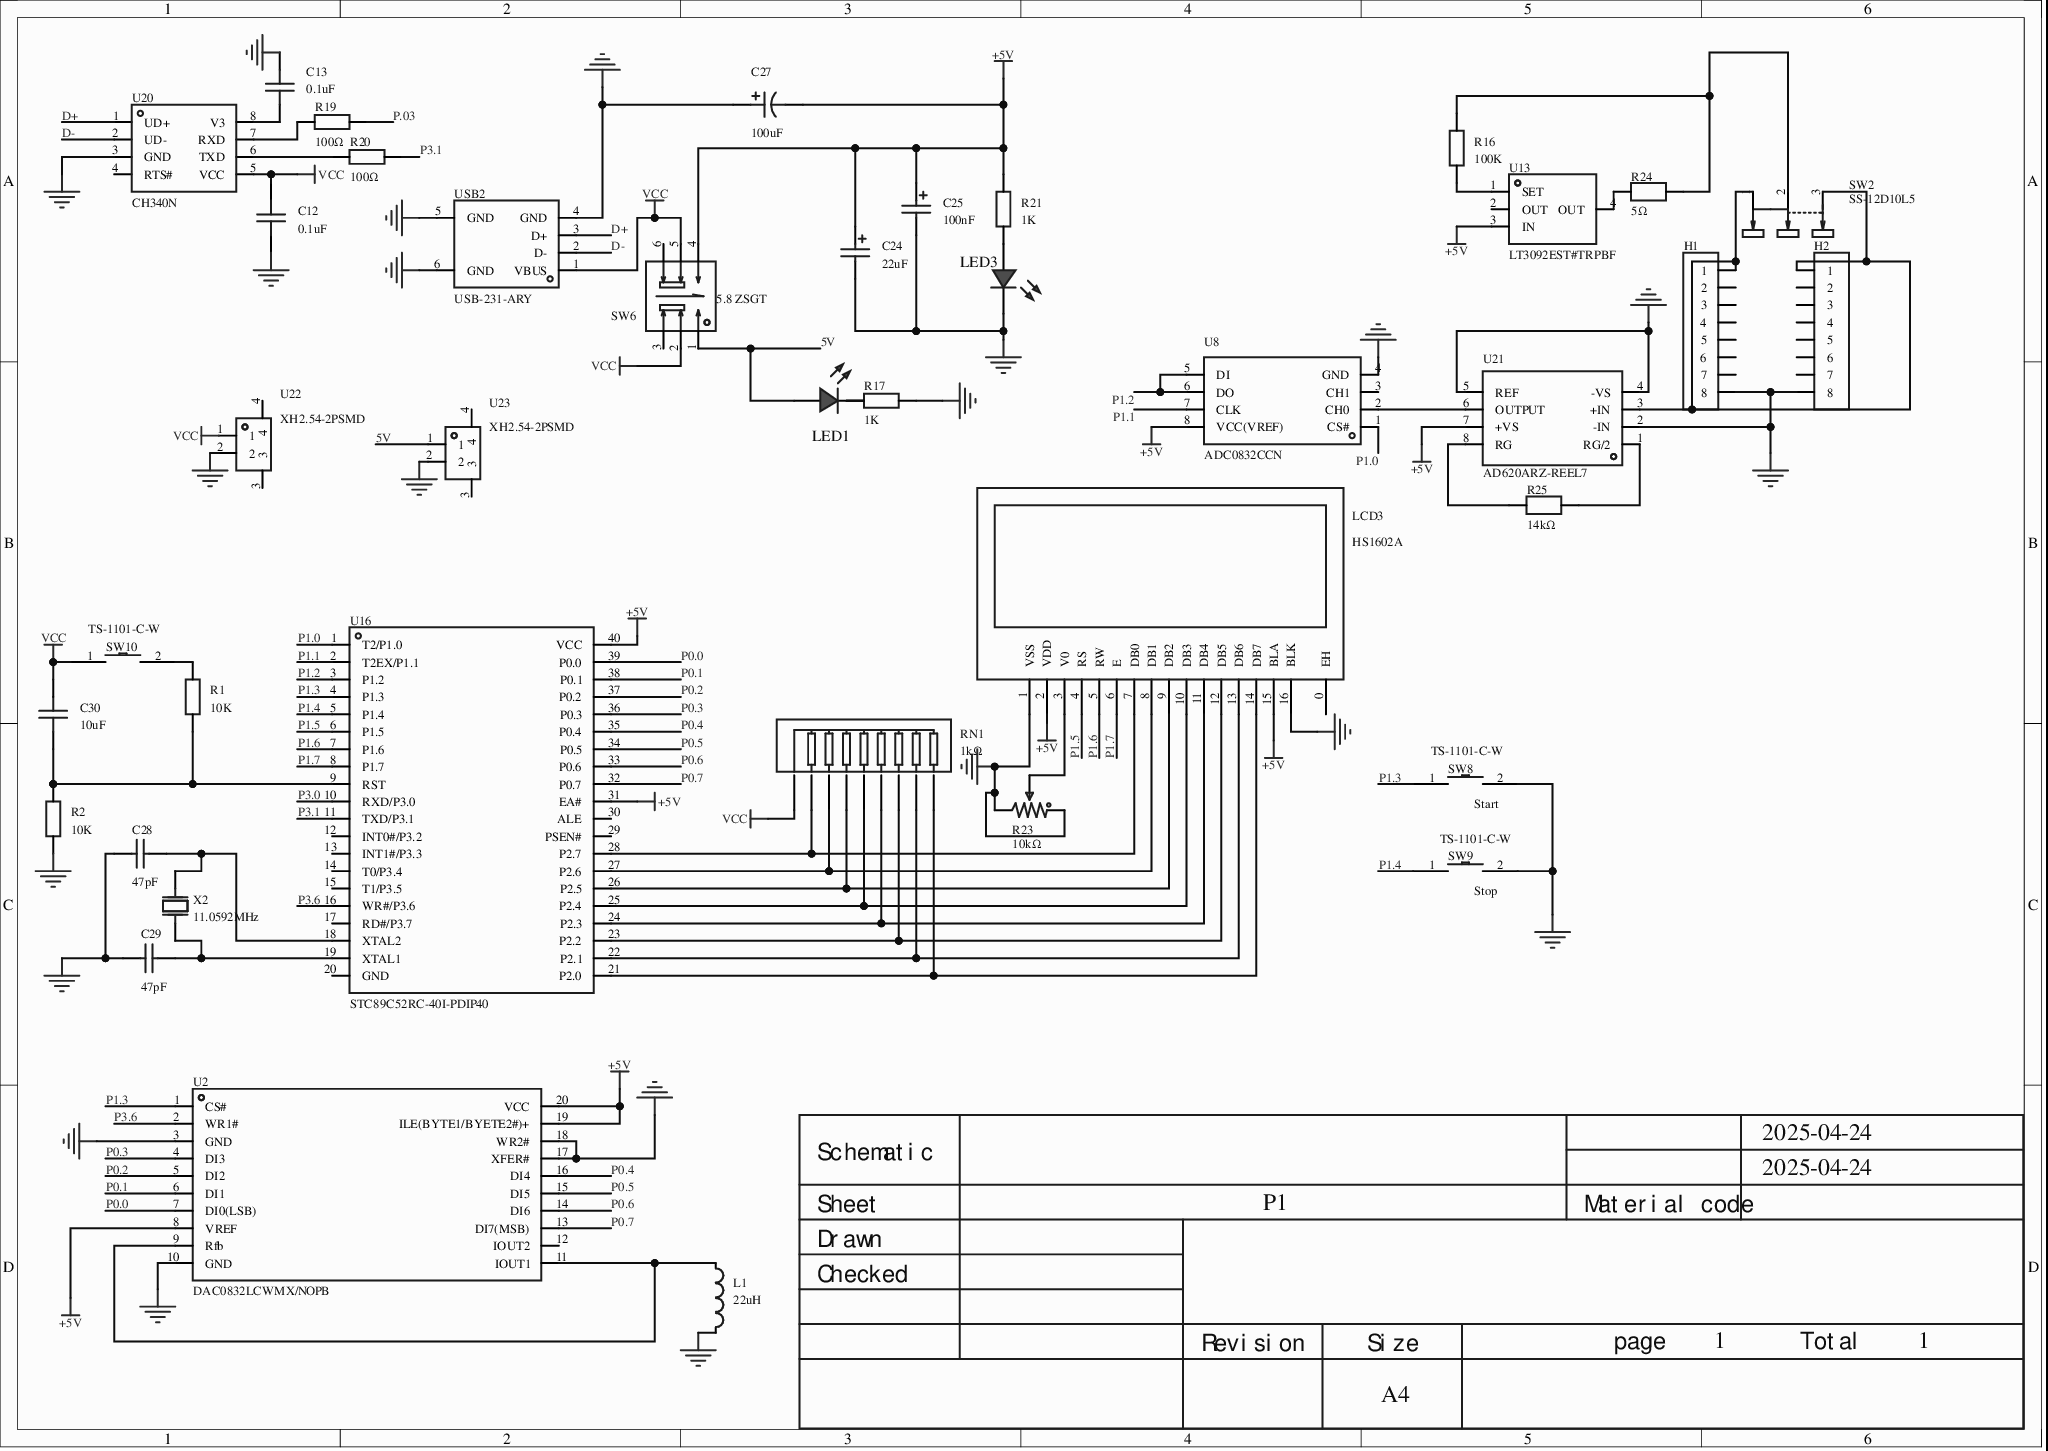
[diagram p0: MISC52088-3.schdoc]
# Altium project MISC52088-2.PrjPcb
1 sheet, 40 parts. Net scope: global (net labels, ports and power ports of the same name join across sheets).
Board file: MISC52088.pcbdoc

## Sheet MISC52088-3.schdoc
size 297 x 210 mm; Version: V1.0; @Project Name: MISC52088; @Page Count: 1; @Update Date: 2025-04-24; @Create Date: 2025-04-24; @Schematic Name: MISC52088; @Page No: 1; @Board Name: MISC52088; @Create Time: 22:25:30; @Update Time: 22:26:05

### Parts
C12  0.1uF  [C0603]
C13  0.1uF  [C0603]
C24  22uF  [CAP-SMD_L3.5-W2.8-R-RD]
C25  100nF  [CASE-A_3216]
C27  100uF  [CAP-SMD_BD8.1-L8.3-W8.3-LS9.3-FD]
C28  47pF  [C0603]
C29  47pF  [C0603]
C30  10uF  [C0603]
H1  (no value)  [HDR-TH_8P-P2.54-V-F-1]
H2  (no value)  [HDR-TH_8P-P2.54-V-F-1]
L1  22uH  [IND-TH_BD14.7-2P-P4.00]
LCD3  HS1602A  [LCD1602]
LED1  (no value)  [LED_0603]
LED3  (no value)  [LED_0603]
R1  10K  [R0603]
R2  10K  [R0603]
R16  100K  [R0603]
R17  1K  [R0603]
R19  100Ω  [R0603]
R20  100Ω  [R0603]
R21  1K  [R0603]
R23  10kΩ  [RES-ADJ-SMD_3P-L3.0-W3.8-P1.75-BR]
R24  5Ω  [R2512]
R25  14kΩ  [R0603]
RN1  1kΩ  [RES-ARRAY-TH_9P-P2.54-D1.0]
SW2  SS-12D10L5  [SW-TH_SS-12D10L5]
SW6  5.8 ZSGT  [SW-TH_5.8ZSGT]
SW8  TS-1101-C-W  [SW-SMD_L6.0-W3.3-LS8.0]
SW9  TS-1101-C-W  [SW-SMD_L6.0-W3.3-LS8.0]
SW10  TS-1101-C-W  [SW-SMD_L6.0-W3.3-LS8.0]
U2  DAC0832LCWMX/NOPB  [SOIC-20_L13.0-W7.6-P1.27-LS10.3-BL]
U8  ADC0832CCN  [DIP-8_L9.7-W6.4-P2.54-LS7.6-BL]
U13  LT3092EST#TRPBF  [SOT-223-4_L6.5-W3.5-P2.30-LS7.0-BR]
U16  STC89C52RC-40I-PDIP40  [DIP-40_L52.0-W13.7-P2.54-LS15.2-BL]
U20  CH340N  [SOP-8_L4.9-W3.9-P1.27-LS6.0-BL]
U21  AD620ARZ-REEL7  [SOIC-8_L5.0-W4.0-P1.27-LS6.0-BL]
U22  XH2.54-2PSMD  [CONN-SMD_XH2.54-2PSMD]
U23  XH2.54-2PSMD  [CONN-SMD_XH2.54-2PSMD]
USB2  USB-231-ARY  [USB-A-TH_USB-231-ARY]
X2  11.0592MHz  [HC-49US_L11.5-W4.5-P4.88]

### Nets
+5V: C24.1 C25.1 C27.2 LCD3.2(VDD) LCD3.15(BLA) R21.2 SW6.4 U2.8(VREF) U2.19(ILE(BYTE1/BYETE2#)+) U2.20(VCC) U8.8(VCC(VREF)) U13.3(IN) U16.31(EA#) U16.40(VCC) U21.7(+VS)
GND: C12.1 C13.1 C24.2 C25.2 C27.1 C28.1 C29.1 H1.8 H2.8 L1.2 LCD3.1(VSS) LCD3.16(BLK) LED3.1(C) R2.1 R17.2 R23.1 R23.3 SW8.2 SW9.2 U2.3(GND) U2.10(GND) U2.17(XFER#) U2.18(WR2#) U8.4(GND) U20.3(GND) U21.2(-IN) U21.4(-VS) U21.5(REF) U22.2 U23.2 USB2.4(GND) USB2.5(GND) USB2.6(GND)
VCC: C12.2 C30.2 RN1.1 SW6.2 SW6.5 SW10.1 U20.5(VCC) U22.1 USB2.1(VBUS)
5V: LED1.2(A) SW6.1 U23.1
D+: U20.1(UD+) USB2.3(D+)
D-: U20.2(UD-) USB2.2(D-)
P0.0: U2.7(DI0(LSB)) U16.39(P0.0)
P0.1: U2.6(DI1) U16.38(P0.1)
P0.2: U2.5(DI2) U16.37(P0.2)
P0.3: U2.4(DI3) U16.36(P0.3)
P0.4: U2.16(DI4) U16.35(P0.4)
P0.5: U2.15(DI5) U16.34(P0.5)
P0.6: U2.14(DI6) U16.33(P0.6)
P0.7: U2.13(DI7(MSB)) U16.32(P0.7)
P1.0: U8.1(CS#) U16.1(T2/P1.0)
P1.1: U8.7(CLK) U16.2(T2EX/P1.1)
P1.2: U8.5(DI) U8.6(DO) U16.3(P1.2)
P1.3: SW8.1 U2.1(CS#) U16.4(P1.3)
P1.4: SW9.1 U16.5(P1.4)
P1.5: LCD3.4(RS) U16.6(P1.5)
P1.6: LCD3.5(RW) U16.7(P1.6)
P1.7: LCD3.6(E) U16.8(P1.7)
P3.0: U16.10(RXD/P3.0)
P3.1: R20.2 U16.11(TXD/P3.1)
P3.6: U2.2(WR1#) U16.16(WR#/P3.6)
P.03: R19.2
NetC13_2: C13.2 U20.8(V3)
NetC28_2: C28.2 U16.18(XTAL2) X2.1(OSC1)
NetC29_2: C29.2 U16.19(XTAL1) X2.2(OSC2)
NetC30_1: C30.1 R1.1 R2.2 U16.9(RST)
NetH1_1: H1.1 H2.1 SW2.1 SW2.3 U21.3(+IN)
NetL1_1: L1.1 U2.9(Rfb) U2.11(IOUT1)
NetLCD3_3: LCD3.3(V0) R23.2
NetLCD3_7: LCD3.7(DB0) RN1.2 U16.28(P2.7)
NetLCD3_8: LCD3.8(DB1) RN1.3 U16.27(P2.6)
NetLCD3_9: LCD3.9(DB2) RN1.4 U16.26(P2.5)
NetLCD3_10: LCD3.10(DB3) RN1.5 U16.25(P2.4)
NetLCD3_11: LCD3.11(DB4) RN1.6 U16.24(P2.3)
NetLCD3_12: LCD3.12(DB5) RN1.7 U16.23(P2.2)
NetLCD3_13: LCD3.13(DB6) RN1.8 U16.22(P2.1)
NetLCD3_14: LCD3.14(DB7) RN1.9 U16.21(P2.0)
NetLED1_1: LED1.1(C) R17.1
NetLED3_2: LED3.2(A) R21.1
NetR1_2: R1.2 SW10.2
NetR16_1: R16.1 U13.1(SET)
NetR16_2: R16.2 R24.2 SW2.2
NetR19_1: R19.1 U20.7(RXD)
NetR20_1: R20.1 U20.6(TXD)
NetR24_1: R24.1 U13.4(OUT)
NetR25_1: R25.1 U21.8(RG)
NetR25_2: R25.2 U21.1(RG/2)
NetU8_2: U8.2(CH0) U21.6(OUTPUT)

Not connected (* = marked no-connect by the designer): H1 2 3 4 5 6 7; H2 2 3 4 5 6 7; LCD3 0(EH); SW6 3 6; U2 12(IOUT2); U8 3(CH1); U13 2(OUT); U16 12(INT0#/P3.2) 13(INT1#/P3.3) 14(T0/P3.4) 15(T1/P3.5) 17(RD#/P3.7) 20(GND) 29(PSEN#) 30(ALE); U20 4(RTS#); U22 3 4; U23 3 4

### Notes on the sheet
- (near SW8) Start
- (near SW9) Stop
- 2025-04-24
- Schematic
- Sheet
- P1
- Material code
- Checked
- Drawn
- Revision
- Size
- A4
- page
- 1
- Total

### Library data of the parts
C12 C13 = CAP_0603: ConvertToPcb: yes; SymbolName: CapAcitance; ModelId: ac125912035d415993ca9572d50418b1; ModelName: C0603_L1.6-W0.8-H0.8; ModelTransform: 62.992,31.496,0,0,0,0,0,0,0; Value: 100nF; Device: CAP_0603; AddInBom: yes; Supplier Footprint: 0603; FootprintName: C0603
C24 = 6TPE220MAZB: Capacitance: 220uF; tolerance: ±20%; rated voltage: 6.3V; equivalent series resistance (ESR): 35mΩ@100kHz;; Manufacturer: PANASONIC(松下); AddInBom: yes; ModelId: 0dfcda272f9b43668c6086d3a08712ba; ModelName: CASE-B_L3.5-W2.8-H1.9; ModelTransform: 145.669,110.236,0,180,0,0,0,0,0; Symbol: 6TPE220MAZB; Value: 22uF; Device: 6TPE220MAZB; LCSC Part Name: 220uF ±20% 6.3V MSL=3拆包后请尽快使用; ManufacturerPart: 6TPE220MAZB; Supplier Footprint: -; JLCPCB Part Class: Extended library; Datasheet: https://atta.szlcsc.com/upload/public/pdf/source/20180301/C178383_15198943937361383951.pdf; Supplier: LCSC; ConvertToPcb: yes; FootprintName: CAP-SMD_L3.5-W2.8-R-RD; Tolerance: ±20%; Voltage Rating: 6.3V; Equivalent Series Resistance(ESR): 35mΩ@100kHz; Operating Temperature: -55℃~+105℃
C25 = TAJA104K035RNJ: Capacitance: 100nF; tolerance: ±10%; rated voltage: 35V; equivalent series resistance: 24Ω@100kHz;; Manufacturer: Kyocera AVX; AddInBom: yes; ModelId: 803ac3def75e4c7cb895540fe23dd6a1; ModelTransform: 125.984,62.992,0,0,0,0,0,0,0; Symbol: TAJA104K035RNJ; Device: TAJA104K035RNJ; LCSC Part Name: 100nF ±10% 35V; SupplierPart: C7173; ManufacturerPart: TAJA104K035RNJ; Supplier Footprint: CASE-A-3216; JLCPCB Part Class: Extended library; Datasheet: https://atta.szlcsc.com/upload/public/pdf/source/20160107/1457707750344.pdf; Supplier: LCSC; ConvertToPcb: yes; FootprintName: CASE-A_3216; ModelName: CASE-A_3216; Value: 100nF; Tolerance: ±10%; Rated Voltage: 35V; Equivalent Series Resistance(ESR): 24Ω@100kHz; Operating Temperature: -55℃~+125℃
C27 = GVE1H107M0810CNVC: Capacitance: 100uF; tolerance: ±20%; rated voltage: 50V; ripple current: 300mA@100kHz; equivalent series resistance: 600mΩ@100kHz;; Manufacturer: HRK(鸿瑞凯电子); AddInBom: yes; ModelId: 42ed741c1b0b4e9db37bf14bd0fb5205; ModelTransform: 354.33,326.771,0,180,0,0,0,0,0; φD: 8mm; L: 10.5mm; Lifetime @ Temp: 2000hrs@105℃; Symbol: GVE1H107M0810CNVC; Device: GVE1H107M0810CNVC; LCSC Part Name: 100uF ±20% 50V; SupplierPart: C2983307; ManufacturerPart: GVE1H107M0810CNVC; Supplier Footprint: SMD,D8xL10.5mm; JLCPCB Part Class: Extended library; Datasheet: https://atta.szlcsc.com/upload/public/pdf/source/20220321/B5A059027F69866A3EEEBC781A889613.pdf; Supplier: LCSC; ConvertToPcb: yes; FootprintName: CAP-SMD_BD8.1-L8.3-W8.3-LS9.3-FD; ModelName: CAP-SMD_BD8.1-L8.3-W8.3-LS9.3-FD; Value: 100uF; Tolerance: ±20%; Rated Voltage: 50V; Ripple Current: 300mA@100kHz; Equivalent Series Resistance(ESR): 600mΩ@100kHz; Operating Temperature: -55℃~+105℃
C28 C29 = CL10C470JB8NNNC: Capacitance: 47pF; tolerance: ±5%; rated voltage: 50V; dielectric (temperature coefficient): C0G;; Manufacturer: SAMSUNG(三星); AddInBom: yes; ModelId: ac125912035d415993ca9572d50418b1; ModelName: C0603_L1.6-W0.8-H0.8; ModelTransform: 62.992,31.496,0,0,0,0,0,0,0; Symbol: CL10C470JB8NNNC; Device: CL10C470JB8NNNC; LCSC Part Name: 47pF ±5% 50V; SupplierPart: C1671; ManufacturerPart: CL10C470JB8NNNC; Supplier Footprint: 0603; JLCPCB Part Class: Basic library; Datasheet: https://atta.szlcsc.com/upload/public/pdf/source/20160218/1457707763339.pdf; Supplier: LCSC; ConvertToPcb: yes; FootprintName: C0603; Value: 47pF; Tolerance: ±5%; Voltage Rated: 50V; Temperature Coefficient: C0G
C30 = CGA0603X5R106K100JT: Capacitance: 10uF; tolerance: ±10%; rated voltage: 10V; temperature coefficient: X5R;; Manufacturer: HRE(芯声); AddInBom: yes; ModelId: ac125912035d415993ca9572d50418b1; ModelName: C0603_L1.6-W0.8-H0.8; ModelTransform: 62.992,31.496,0,0,0,0,0,0,0; Symbol: CGA0603X5R106K100JT; Device: CGA0603X5R106K100JT; LCSC Part Name: 10uF ±10% 10V; SupplierPart: C6119842; ManufacturerPart: CGA0603X5R106K100JT; Supplier Footprint: 0603; JLCPCB Part Class: Extended library; Supplier: LCSC; ConvertToPcb: yes; FootprintName: C0603; Value: 10uF; Tolerance: ±10%; Voltage Rating: 10V; Temperature Coefficient: X5R
H1 H2 = HDR-F_2.54_1x8P: Symbol: Header-Female-2.54_1x8; AddInBom: yes; ModelId: 0f7e4d9227ef4fa08d5469c22cc70cdb; ModelName: HDR-F-2.54_1x8; ModelTransform: 799.99844,100,0,0,0,0,0,0,-118.11; Device: HDR-F_2.54_1x8P; ConvertToPcb: yes; FootprintName: HDR-TH_8P-P2.54-V-F-1; SupplierPart: C27438; Supplier Footprint: 插件
L1 = PDMTAT044125-220MWU: Inductance: 22uH; tolerance: ±20%; rated current: 8A; saturation current (Isat): -; type: toroidal inductor; Q factor: -;; Manufacturer: PROD(谱罗德); AddInBom: yes; ModelId: ffc1d1e6ac7e4445805eb288369d3ccc; ModelTransform: 578.23735,577.65514,0,0,0,0,0,196.85,-118.11; DC Resistance: 15mΩ; Symbol: PDMTAT044125-220MWU; Device: PDMTAT044125-220MWU; LCSC Part Name: 磁环电感 22uH ±20%; SupplierPart: C2909799; ManufacturerPart: PDMTAT044125-220MWU; Supplier Footprint: 插件,D=14.5mm; JLCPCB Part Class: Extended library; Datasheet: https://atta.szlcsc.com/upload/public/pdf/source/20211105/260D4E3EA41F790233DE2825ED13716B.pdf; Supplier: LCSC; ConvertToPcb: yes; FootprintName: IND-TH_BD14.7-2P-P4.00; ModelName: IND-TH_BD14.7-2P-P4.00; Value: 22uH; Tolerance: ±20%; Rated Current: 8A; Current - Saturation (Isat): -; Type: Toroidal inductor; Q @ Frequency: -; Frequency - Self Resonant: -; Ratings: AEC-Q200
LCD3 = HS1602A: Controller chip: SPLC780; size (inch): 2;; Manufacturer: HS(汉昇); AddInBom: yes; ModelId: f9d832f46a914cadb50fc4d4cefd2517; ModelTransform: 3149.6,1417.32,0,0,0,0,0,0,-118.11; Symbol: HS1602A; Device: HS1602A; LCSC Part Name: 2.0寸16*2单色字符字符液晶显示屏; SupplierPart: C5329588; ManufacturerPart: HS1602A; Supplier Footprint: -; JLCPCB Part Class: Extended library; Datasheet: https://atta.szlcsc.com/upload/public/pdf/source/20221212/35734F14DBB323F90DD8DBE1717CD9FD.pdf; Supplier: LCSC; ConvertToPcb: yes; FootprintName: LCD1602; ModelName: LCD1602; Main Control Chip: SPLC780; Size: 2; Operating Temperature: -20℃~+70℃
LED1 LED3 = LED_0603-R: Symbol: LED_R; Convert to PCB: yes; 3D Model: dd8257b0d61a4cd7b68939a056e08095; 3D Model Transform: 58.72,29.4,22.03,0,0,0,0,0,0; ModelName: LED-0603_R; Device: LED_0603-R; Add into BOM: yes; Supplier Footprint: 0603; FootprintName: LED_0603
R1 R2 R21 = Res_0603: ConvertToPcb: yes; SymbolName: Resistor; ModelId: fc143cca1e79419f9cd78b61e9279f08; ModelTransform: 31.8897,63.7794,0,90,0,0,0,0,0; Device: Res_0603; AddInBom: yes; Supplier Footprint: 0603; FootprintName: R0603; ModelName: R0603
  R1 R2: Value: 10K
  R21: Value: 1K
R16 R17 R19 R20 = Res_0603: ConvertToPcb: yes; SymbolName: Resistor; ModelId: fc143cca1e79419f9cd78b61e9279f08; ModelTransform: 31.8897,63.7794,0,90,0,0,0,0,0; Value: 10K; Device: Res_0603; AddInBom: yes; Supplier Footprint: 0603; FootprintName: R0603; ModelName: R0603
R23 = TC33X-2-103E: Resistance: 10kΩ; tolerance: ±25%; power: 150mW; temperature coefficient: ±250ppm/℃;; Manufacturer: BOURNS; AddInBom: yes; ModelId: 6fe475bd84584852aea8190beccbfb0a; ModelTransform: 118.11,150,0,90,0,0,4.882,0,0; Turns: 1; Symbol: TC33X-2-103E; Device: TC33X-2-103E; LCSC Part Name: 10kΩ ±25%; SupplierPart: C719176; ManufacturerPart: TC33X-2-103E; Supplier Footprint: SMD-3P,3.8x3.6mm; JLCPCB Part Class: Extended library; Datasheet: https://atta.szlcsc.com/upload/public/pdf/source/20200810/C720646_BB66A75E654D5E1D30127FF45BCD3C26.pdf; Supplier: LCSC; ConvertToPcb: yes; FootprintName: RES-ADJ-SMD_3P-L3.0-W3.8-P1.75-BR; ModelName: RES-ADJ-SMD_3P-L3.0-W3.8-P1.75-BR; Value: 10kΩ; Tolerance: ±25%; Rated Voltage: -; Power(Watts): 150mW; Temperature Coefficient: ±250ppm/℃
R24 = HoAR2512-1W-5R-0.1%-TCR25: Resistor type: ceramic resistor; resistance: 5Ω; tolerance: ±0.1%; power: 1W; temperature coefficient: ±25ppm/℃;; Manufacturer: Milliohm(毫欧); AddInBom: yes; ModelId: 954b67263d9e4f3582d8de3f8c846421; ModelName: R2512_L6.3-W3.2-H0.6; ModelTransform: 248.031,125.984,0,0,0,0,-0.0005,0,0; Symbol: HOAR2512-1W-5R-0.1%-TCR25; Device: HoAR2512-1W-5R-0.1%-TCR25; LCSC Part Name: 陶瓷电阻 5Ω ±0.1% 1W; SupplierPart: C5123609; ManufacturerPart: HoAR2512-1W-5R-0.1%-TCR25; Supplier Footprint: 2512; JLCPCB Part Class: Extended library; Datasheet: https://atta.szlcsc.com/upload/public/pdf/source/20220805/BC8894D01B21B12D20FF0E940066DD50.pdf; Supplier: LCSC; ConvertToPcb: yes; FootprintName: R2512; Type: Ceramic resistor; Value: 5Ω; Tolerance: ±0.1%; Power(Watts): 1W; Temperature Coefficient: ±25ppm/℃
R25 = FRC0603F1402TS: Resistor type: thick-film resistor; resistance: 14kΩ; tolerance: ±1%; power: 100mW; operating voltage: 75V; temperature coefficient: ±100ppm/℃;; Manufacturer: FOJAN(富捷); AddInBom: yes; ModelId: fc143cca1e79419f9cd78b61e9279f08; ModelTransform: 31.8897,63.7794,0,90,0,0,0,0,0; Symbol: FRC0603F1402TS; Device: FRC0603F1402TS; LCSC Part Name: 14kΩ ±1% 100mW 厚膜电阻; SupplierPart: C2930066; ManufacturerPart: FRC0603F1402TS; Supplier Footprint: 0603; JLCPCB Part Class: Extended library; Datasheet: https://atta.szlcsc.com/upload/public/pdf/source/20211221/925EC7D7225764EE0046F22065062C87.pdf; Supplier: LCSC; ConvertToPcb: yes; FootprintName: R0603; ModelName: R0603; Type: Thick-film resistor; Value: 14kΩ; Tolerance: ±1%; Power(Watts): 100mW; Voltage-Supply(Max): 75V; Temperature Coefficient: ±100ppm/℃; Operating Temperature: -55℃~+155℃
RN1 = A09-102JP: Number of resistors: 8; resistance: 1kΩ; tolerance: ±5%; power per element: 125mW; temperature coefficient: ±100ppm/℃;; Manufacturer: FH(风华); AddInBom: yes; ModelId: d106c67f29e14d8080ba548247a719a1; ModelName: SIP-9_L22.8-W3.0-H8.5-P2.54; ModelTransform: 917.49722,118.11,0,0,0,0,0,0,-137.795; Number of Resistors: 8; Symbol: A09-102JP; Device: A09-102JP; LCSC Part Name: 1kΩ ±5%; SupplierPart: C9111; ManufacturerPart: A09-102JP; Supplier Footprint: SIP-9-2.54mm; JLCPCB Part Class: Extended library; Datasheet: https://atta.szlcsc.com/upload/public/pdf/source/20181127/C336620_2E84FA9E7B5BF76546BC661699514FB8.pdf; Supplier: LCSC; ConvertToPcb: yes; FootprintName: RES-ARRAY-TH_9P-P2.54-D1.0; Value: 1kΩ; Tolerance: ±5%; Power(Watts): 125mW; Temperature Coefficient: ±100ppm/℃; Number of Pins: 9
SW2 = SS-12D10L5: Circuit structure: SPDT; mounting: through-hole; switch colour: black; rated current (DC): 3A; rated voltage (DC): 125V; rated current (AC): 3A; rated voltage (AC): 125V; mechanical life: 1 ten-thousand cycles;; Manufacturer: XKB Connectivity(中国星坤); AddInBom: yes; ModelId: c49f07a32c154ec8ad7cf47670a53981; ModelName: SW-TH_L13.0-W6.8-H6.4-P4.7; ModelTransform: 511.81,267.716,0,0,0,0,0,0,-275.591; Actuator Style: Rectangular post; Pin Style: PC pin; Switch Length: 13mm; Switch Width: 6.8mm; Switch Height: 6.4mm; Symbol: SS-12D10L5; Device: SS-12D10L5; LCSC Part Name: 柄长5mm 直插双档 滑动开关; SupplierPart: C319012; ManufacturerPart: SS-12D10L5; Supplier Footprint: 插件; JLCPCB Part Class: Extended library; Datasheet: https://atta.szlcsc.com/upload/public/pdf/source/20211009/D6412F37AABE6F9459A6EE7FA4DAEADB.pdf; Supplier: LCSC; ConvertToPcb: yes; FootprintName: SW-TH_SS-12D10L5; Circuit: SPDT; Mounting Style: Through-hole; Actuator Color: Black; Current Rating (DC): 3A; Voltage Rating (DC): 125V; Current Rating (AC): 3A; Voltage Rating (AC): 125V; Mechanical Life: 1 ten-thousand cycles; Operating Temperature: -40℃~+85℃
SW6 = 5.8 ZSGT: Circuit structure: DPDT; self-lock / no-lock: self-lock; mounting: through-hole; contact current: 110mA; rated voltage (DC): 30V; with lamp: without; actuating force: 1.5N; mechanical life: 10 ten-thousand cycles;; Manufacturer: SHOU HAN(首韩); AddInBom: yes; ModelId: 3b6e980975cd43bda015b2e9aaa869d3; ModelTransform: 228.346,228.346,0,0,0,0,0,0,-141.732; Actuator Style: Square button; Insulation Resistance: 100MΩ; Actuator/Cap Color: White; Pin Style: PC pin; Symbol: 5.8 ZSGT; Device: 5.8 ZSGT; LCSC Part Name: 5.8*5.8有头/高头 带锁/自锁开关 泡泡机开关; SupplierPart: C2681587; ManufacturerPart: 5.8 ZSGT; Supplier Footprint: 插件; JLCPCB Part Class: Extended library; Datasheet: https://atta.szlcsc.com/upload/public/pdf/source/20210107/C2681587_CDDDDA4A1C7AC9FEB01815B75893A6BA.pdf; Supplier: LCSC; ConvertToPcb: yes; FootprintName: SW-TH_5.8ZSGT; ModelName: SW-TH_5.8ZSGT; Circuit: DPDT; Self Lock / No Lock: Self-lock; Mounting Style: Through-hole; Contact Current: 110mA; Voltage Rating (DC): 30V; With Lamp: Without; Operating Force: 1.5N; Operating Temperature: -10℃~+70℃; Mechanical Life: 10 ten-thousand cycles
SW8-SW10 = TS-1101-C-W: Circuit structure: SPST; button shape: rectangular button; actuating force: 260gf; mounting: surface mount; switch length: 6mm; switch width: 3.6mm; switch height: 2.5mm; with bracket: without; contact current: 50mA; rated voltage (AC): -; rated voltage (DC): 12V; rated power: -; insulation resistance: -; with lamp: none; mechanical life: 5 ten-thousand cycles;; Manufacturer: XKB Connectivity(中国星坤); AddInBom: yes; ModelId: b2f4ea9f0afc4b0786d53dba66ceb9e4; ModelName: SW-SMD_L6.0-W3.3-H5-LS8.0; ModelTransform: 314.96,129.921,0,0,0,0,0,0,0; Actuator/Cap Color: White with light green; Symbol: TS-1101-C-W; Device: TS-1101-C-W; LCSC Part Name: 6*3.6*2.5mm 立贴 轻触开关; SupplierPart: C318938; ManufacturerPart: TS-1101-C-W; Supplier Footprint: SMD; JLCPCB Part Class: Extended library; Datasheet: https://atta.szlcsc.com/upload/public/pdf/source/20200227/C318938_C2E53B1EEDE37D980A33616AC086DE53.pdf; Supplier: LCSC; ConvertToPcb: yes; FootprintName: SW-SMD_L6.0-W3.3-LS8.0; Circuit: SPST; Actuator Style: Rectangular button; Operating Force: 260gf; Mounting Style: Surface mount; Switch Length: 6mm; Switch Width: 3.6mm; Switch Height: 2.5mm; Strike Gundam: Without; Contact Current: 50mA; Voltage Rating (AC): -; Voltage Rating (DC): 12V; Power Rating: -; Insulation Resistance: -; With Lamp: None; IP Rating: -; Pin Style: -; Mechanical Life: 5 ten-thousand cycles; Operating Temperature: -30℃~+85℃
U2 = DAC0832LCWMX/NOPB: Manufacturer: TI(德州仪器); AddInBom: yes; ModelId: fc022553ecdc4755a737d639ae95109c; ModelName: SOIC-20_L12.8-W7.5-H2.7-LS10.3-P1.27; ModelTransform: 503.936,409.68154,0,0,0,0,0,0,0; Symbol: DAC0832LCWMX/NOPB; Device: DAC0832LCWMX/NOPB; LCSC Part Name: DAC0832LCWMX/NOPB; SupplierPart: C17194366; ManufacturerPart: DAC0832LCWMX/NOPB; Supplier Footprint: SOIC-20; JLCPCB Part Class: Extended library; Supplier: LCSC; ConvertToPcb: yes; FootprintName: SOIC-20_L13.0-W7.6-P1.27-LS10.3-BL
U8 = ADC0832CCN_C5357: 8BIT serial A/D converter chip; Manufacturer: ST(意法半导体); AddInBom: yes; ModelId: 5746b540d01a4d1b9eb6b4f989297bc7; ModelName: DIP-8_L9.8-W6.6-H3.5-LS7.62-P2.54; ModelTransform: 385.826,311.8104,0,0,0,0,0,0,-118.11; Symbol: ADC0832CCN_C5357; Device: ADC0832CCN_C5357; LCSC Part Name: ADC0832CCN; SupplierPart: C5357; ManufacturerPart: ADC0832CCN; Supplier Footprint: DIP-8-300mil; JLCPCB Part Class: Extended library; Supplier: LCSC; ConvertToPcb: yes; FootprintName: DIP-8_L9.7-W6.4-P2.54-LS7.6-BL
U13 = LT3092EST#TRPBF: Operating voltage: 1.2V~40V; output current: 200mA;; Manufacturer: ADI(亚德诺); AddInBom: yes; ModelId: 925194bf9823436183a3e0b978a8d076; ModelName: SOT-223-4P_L6.5-W3.5-H1.6-LS7.0-P2.30; ModelTransform: 279.89794,255.905,0,180,0,0,-0.0005,-0.0005,0; Symbol: LT3092EST#TRPBF; Device: LT3092EST#TRPBF; LCSC Part Name: LT3092EST#TRPBF; SupplierPart: C580042; ManufacturerPart: LT3092EST#TRPBF; Supplier Footprint: SOT-223-4; JLCPCB Part Class: Extended library; Datasheet: https://atta.szlcsc.com/upload/public/pdf/source/20191127/C462641_3F8C9FA2233CF5D7421ECCE8C2641F3A.pdf; Supplier: LCSC; ConvertToPcb: yes; FootprintName: SOT-223-4_L6.5-W3.5-P2.30-LS7.0-BR; Type: Current source; Supply Voltage: 1.2V~40V; Output Current: 200mA; Operating Temperature: -40℃~+125℃
U16 = STC89C52RC-40I-PDIP40: CPU core: 51 series; application field: -;; Manufacturer: STC; AddInBom: yes; ModelId: 16d4686a009b4ddca948f91eddb57b14; ModelName: DIP-40_L52.3-W13.8-H4.0-LS15.24-P2.54; ModelTransform: 2059.051,615.743,0,0,0,0,0,0,-118.11; Program Storage Size: 8KB; Program Memory Type: FLASH; Number of I/O: 35; Voltage - Supply: 3.3V~5.5V; Symbol: STC89C52RC-40I; Device: STC89C52RC-40I-PDIP40; LCSC Part Name: STC89C52RC-40I-PDIP40; SupplierPart: C14022; ManufacturerPart: STC89C52RC-40I-PDIP40; Supplier Footprint: DIP-40; JLCPCB Part Class: Extended library; Datasheet: https://atta.szlcsc.com/upload/public/pdf/source/20250219/C2F0DDDE7C5E9ADA5B33742D18630F09.pdf; Supplier: LCSC; ConvertToPcb: yes; FootprintName: DIP-40_L52.0-W13.7-P2.54-LS15.2-BL; CPU Core: 51 series; Applications: -
U20 = CH340N: Application function: USB to serial; interface protocol: USB 2.0; channels: 1; data rate: 2Mbps;; Manufacturer: WCH(南京沁恒); Symbol: CH340N_C2977777; AddInBom: yes; ModelId: 75c24a7891ee4dd6bdac16a7163ff87e; ModelName: SOP-8_L4.9-W3.9-P1.27-LS6.0-BL-1; ModelTransform: 192.913,236.22,0,0,0,0,0,0,0; Protocol: USB 2.0; Number of Channels: 1; Voltage - Supply: 3.3V; 5V; Device: CH340N; LCSC Part Name: USB2.0芯片CH340; SupplierPart: C2977777; ManufacturerPart: CH340N; Supplier Footprint: SOP-8; JLCPCB Part Class: Extended library; Datasheet: https://atta.szlcsc.com/upload/public/pdf/source/20240313/115CDE92081B1D6CB446704AD5D0F5F2.pdf; Supplier: LCSC; ConvertToPcb: yes; FootprintName: SOP-8_L4.9-W3.9-P1.27-LS6.0-BL; Applications Function: USB to serial; Data Rate: 2Mbps; Operating Temperature: -20℃~+70℃
U21 = AD620ARZ-REEL7: Number of amplifiers: single; input bias current (Ib): 500pA; input offset voltage (Vos): 30uV; gain-bandwidth product (GBP): -; slew rate (SR): 1.2V/us; bandwidth (-3db): 1MHz;; Manufacturer: ADI(亚德诺); AddInBom: yes; ModelId: e81d2f7d937b4a6ab1dca543ff5d56a4; ModelName: SOIC-8_L4.9-W3.9-H1.7-LS6.0-P1.27; ModelTransform: 189.751,236.22,0,0,0,0,-0.0005,0.0005,0; Symbol: AD620ARZ-REEL; Device: AD620ARZ-REEL7; LCSC Part Name: 低成本低功耗仪表放大器; SupplierPart: C9675; ManufacturerPart: AD620ARZ-REEL7; Supplier Footprint: SOIC-8; JLCPCB Part Class: Extended library; Datasheet: https://atta.szlcsc.com/upload/public/pdf/source/20121103/1457706545320.pdf; Supplier: LCSC; ConvertToPcb: yes; FootprintName: SOIC-8_L5.0-W4.0-P1.27-LS6.0-BL; Number of Circuits: Single; Current - Input Bias(Ib): 500pA; Voltage - Input Offset(Vos): 30uV; Gain Bandwidth Product(GBP): -; Slew Rate(SR): 1.2V/us; -3db Bandwidth: 1MHz; Operating Temperature: -40℃~+85℃
U22 U23 = XH2.54-2PSMD: AddInBom: yes; ModelId: 014df25e315446289687176395612a56; ModelTransform: 388.9756,411.26571,0,0,0,0,0,5.945,0; Symbol: XH2.54-2PSMD; Device: XH2.54-2PSMD; LCSC Part Name: XH2.54-2PSMD; SupplierPart: C9900001015; ManufacturerPart: XH2.54-2PSMD; Supplier Footprint: XH2.54-2P; JLCPCB Part Class: Extended library; Supplier: LCSC; ConvertToPcb: yes; FootprintName: CONN-SMD_XH2.54-2PSMD; ModelName: CONN-SMD_XH2.54-2PSMD
USB2 = USB-231-ARY: Connector type: Type-A; standard: USB 2.0; gender: female; number of ports: 1; number of contacts: 4P; mounting: right-angle through-hole; rated current - power: 1.5A; contact material: -; contact plating: -; operating temperature range: -20℃~+70℃; soldering temperature (max): 260℃;; Manufacturer: XUNPU(讯普); AddInBom: yes; ModelId: 2c22904cfa634797a8992a7288a8f253; ModelTransform: 610.18209,551.18,0,0,0,0,0,-183.071,-137.795; Number of Ports: 1; Symbol: USB-231-ARY; Device: USB-231-ARY; LCSC Part Name: Type-A 母 弯插; SupplierPart: C720525; ManufacturerPart: USB-231-ARY; Supplier Footprint: 插件; JLCPCB Part Class: Extended library; Datasheet: https://atta.szlcsc.com/upload/public/pdf/source/20200810/C720525_A4C9C15D608FF9239C9C137FD959DB52.pdf; Supplier: LCSC; ConvertToPcb: yes; FootprintName: USB-A-TH_USB-231-ARY; ModelName: USB-A-TH_USB-231-ARY; Connector Type: Type-A; Standard: USB 2.0; Gender: Female; Number of Contacts: 4P; Mounting Style: Right-angle through-hole; Current Rating - Power (Max): 1.5A; Contact Material: -; Contact Plating: -; Operating Temperature Range: -20℃~+70℃; Soldering Temperature(Max): 260℃
X2 = X49SD110592MSD2SC: Crystal type: through-hole crystal; frequency: 11.0592MHz; room-temperature tolerance: ±20ppm; load capacitance: 20pF; frequency stability: ±30ppm;; Manufacturer: YXC(扬兴晶振); AddInBom: yes; ModelId: a8e34f6c394c4d60ace7720f62d1ccdf; ModelName: HC-49US_L11.0-W4.5-H3.5-P4.88; ModelTransform: 432.46488,177.165,0,0,0,0,0,0,-137.795; Symbol: X49SD110592MSD2SC; Device: X49SD110592MSD2SC; LCSC Part Name: 11.0592MHz ±20ppm 20pF; SupplierPart: C2203; ManufacturerPart: X49SD110592MSD2SC; Supplier Footprint: HC-49S; JLCPCB Part Class: Extended library; Datasheet: https://atta.szlcsc.com/upload/public/pdf/source/20240329/977D7F2434F98B2BE33270BB9FF3D86D.pdf; Supplier: LCSC; ConvertToPcb: yes; FootprintName: HC-49US_L11.5-W4.5-P4.88; Type: Through-hole crystal; Value: 11.0592MHz; Normal temperature Frequency Tolerance: ±20ppm; Load Capacitance: 20pF; Frequency Stability: ±30ppm; Operating Temperature: -20℃~+70℃